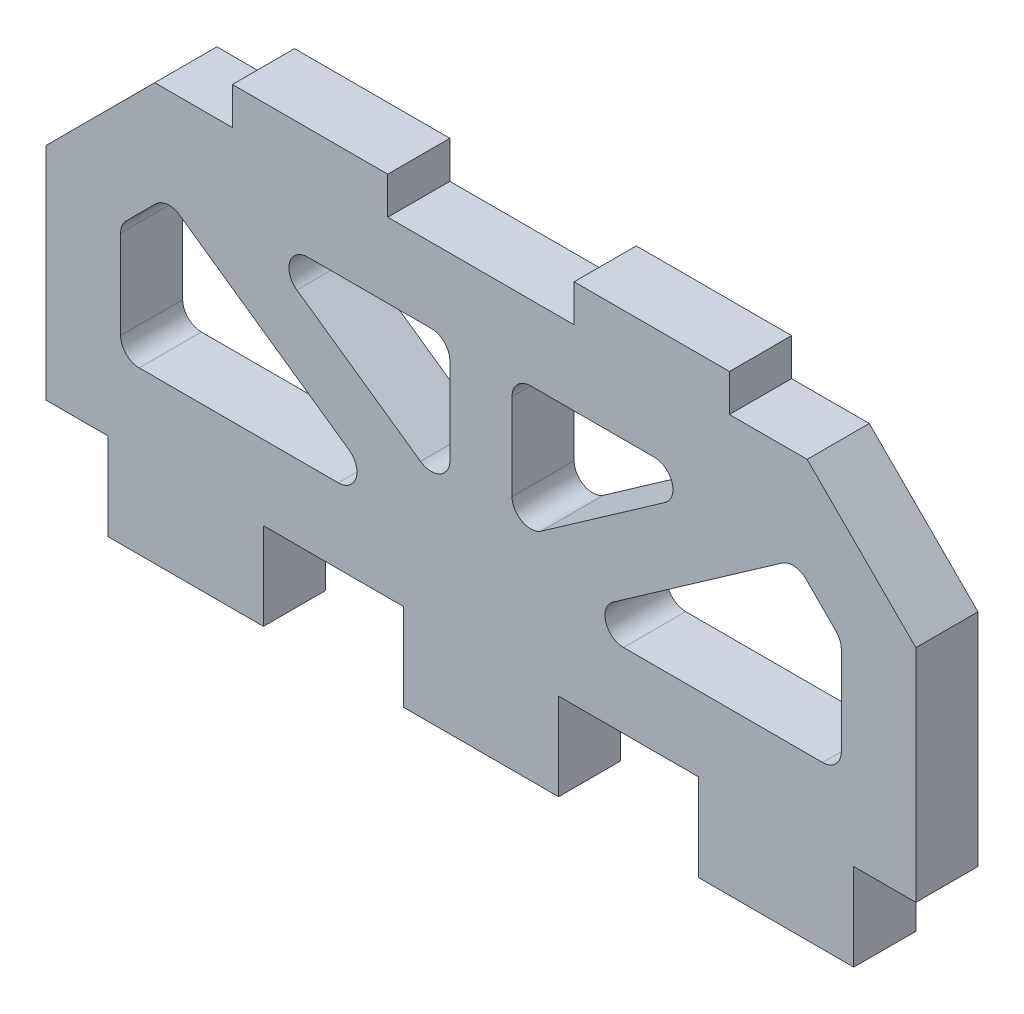
SolidWorks part; units mm, degrees
ref_plane "前视基准面" through (0, 0, 0) normal (0, 0, 1) x (1, 0, 0)
ref_plane "上视基准面" through (0, 0, 0) normal (0, 1, 0) x (1, 0, 0)
ref_plane "右视基准面" through (0, 0, 0) normal (1, 0, 0) x (0, 0, -1)
other "Configuration Table"
sketch "草图1" plane through (0, 0, 0) normal (0, 0, 1) x (1, 0, 0)
  line L0 (0, 61.877) -> (0, -56.8512) construction
  line L1 (-90.5392, 0) -> (103.6937, 0) construction
  line L2 (7.7852, 15.3095) -> (-7.2148, 15.3095)
  line L3 (-7.2148, 15.3095) -> (-7.2148, 18.3095)
  line L4 (-7.2148, 18.3095) -> (-19.7148, 18.3095)
  line L5 (-19.7148, 18.3095) -> (-19.7148, 15.3095)
  line L6 (-19.7148, 15.3095) -> (-25.9648, 15.3095)
  line L7 (-25.9648, 15.3095) -> (-34.7148, 6.5595)
  line L8 (-34.7148, 6.5595) -> (-34.7148, -11.1905)
  line L9 (-34.7148, -11.1905) -> (-29.7148, -11.1905)
  line L10 (-29.7148, -11.1905) -> (-29.7148, -18.2079)
  line L11 (-29.7148, -18.2079) -> (-17.2148, -18.2079)
  line L12 (-17.2148, -18.2079) -> (-17.2148, -11.1905)
  line L13 (-17.2148, -11.1905) -> (-5.9648, -11.1905)
  line L14 (-5.9648, -11.1905) -> (-5.9648, -18.2079)
  line L15 (-5.9648, -18.2079) -> (6.5352, -18.2079)
  line L16 (-24.9876, 7.8013) -> (-28.7148, 4.0742)
  line L17 (-28.7148, 4.0742) -> (-28.7148, -5.1905)
  line L18 (-28.7148, -5.1905) -> (-6.4333, -5.1905)
  line L19 (-6.4333, -5.1905) -> (-24.9876, 7.8013)
  line L20 (-18.4242, 9.3095) -> (-2.2148, 9.3095)
  line L21 (-2.2148, 9.3095) -> (-2.2148, -2.0405)
  line L22 (-2.2148, -2.0405) -> (-18.4242, 9.3095)
  line L23 (2.7852, -2.0405) -> (18.9947, 9.3095)
  line L24 (2.7852, 9.3095) -> (2.7852, -2.0405)
  line L25 (18.9947, 9.3095) -> (2.7852, 9.3095)
  line L26 (7.0038, -5.1905) -> (25.5581, 7.8013)
  line L27 (29.2852, -5.1905) -> (7.0038, -5.1905)
  line L28 (29.2852, 4.0742) -> (29.2852, -5.1905)
  line L29 (25.5581, 7.8013) -> (29.2852, 4.0742)
  line L30 (6.5352, -11.1905) -> (6.5352, -18.2079)
  line L31 (17.7852, -11.1905) -> (6.5352, -11.1905)
  line L32 (17.7852, -18.2079) -> (17.7852, -11.1905)
  line L33 (30.2852, -18.2079) -> (17.7852, -18.2079)
  line L34 (30.2852, -11.1905) -> (30.2852, -18.2079)
  line L35 (35.2852, -11.1905) -> (30.2852, -11.1905)
  line L36 (35.2852, 6.5595) -> (35.2852, -11.1905)
  line L37 (26.5352, 15.3095) -> (35.2852, 6.5595)
  line L38 (20.2852, 15.3095) -> (26.5352, 15.3095)
  line L39 (20.2852, 18.3095) -> (20.2852, 15.3095)
  line L40 (7.7852, 18.3095) -> (20.2852, 18.3095)
  line L41 (7.7852, 15.3095) -> (7.7852, 18.3095)
  point P34 (0.2852, -18.2079)
  point P46 (0.2852, 15.3095)
  dimension "D1" = 7.0173
  dimension "D2" = 11.25
  dimension "D3" = 3
  dimension "D4" = 26.5
  dimension "D5" = 12.5
  dimension "D6" = 12.5
  dimension "D7" = 6
  dimension "D8" = 6
  dimension "D9" = 6
  dimension "D10" = 35
  dimension "D11" = 6
  dimension "D12" = 11.35
  dimension "D13" = 5
extrude "凸台-拉伸1" add sketch "草图1" along normal blind 5
fillet "圆角3" radius 1.5 1 edges at (-24.9876, 7.8013, 2.5)
fillet "圆角4" radius 1.5 3 edges at (-6.4333, -5.1905, 2.5) (-28.7148, -5.1905, 2.5) (-28.7148, 4.0742, 2.5)
fillet "圆角5" radius 1.5 10 edges at (29.2852, -5.1905, 2.5) (29.2852, 4.0742, 2.5) (25.5581, 7.8013, 2.5) (7.0038, -5.1905, 2.5) (18.9947, 9.3095, 2.5) (2.7852, -2.0405, 2.5) (2.7852, 9.3095, 2.5) (-2.2148, -2.0405, 2.5) (-2.2148, 9.3095, 2.5) (-18.4242, 9.3095, 2.5)
